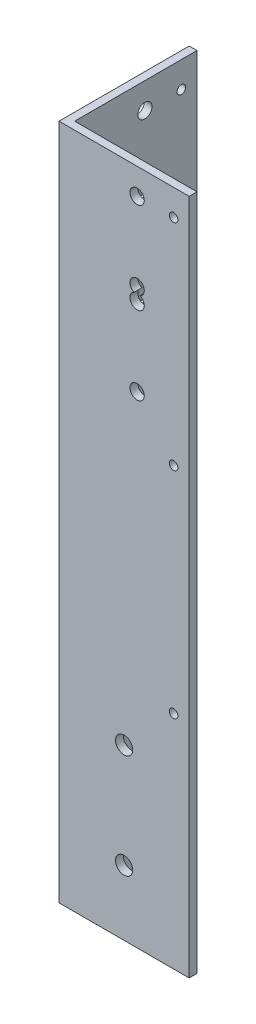
SolidWorks part; units mm, degrees
material "6061Al"
ref_plane "前视基准面" through (0, 0, 0) normal (0, 0, 1) x (1, 0, 0)
ref_plane "上视基准面" through (0, 0, 0) normal (0, 1, 0) x (1, 0, 0)
ref_plane "右视基准面" through (0, 0, 0) normal (1, 0, 0) x (0, 0, -1)
sketch "草图1" plane through (0, 0, 0) normal (0, 1, 0) x (1, 0, 0)
  line L0 (0, 0) -> (50, 0)
  line L1 (0, 0) -> (0, 50)
  line L2 (3, 3) -> (3, 50)
  line L3 (3, 3) -> (50, 3)
  line L4 (0, 50) -> (3, 50)
  line L5 (50, 3) -> (50, 0)
  dimension "D1" = 50
  dimension "D2" = 50
  dimension "D3" = 3
extrude "凸台-拉伸1" add sketch "草图1" along normal blind 260
hole_wizard "M5 间隙孔1" positions "草图2" profile "草图3" hole size "M5" standard "ISO" end condition through all
sketch "草图2" plane through (0, 0, -3) normal (0, 0, -1) x (-1, 0, 0)
  line L0 (-30, 215) -> (-30, 185) construction
  line L1 (-50, 260) -> (-50, 0) construction
  line L2 (-50, 260) -> (-3, 260) construction
  point P0 (-30, 250)
  point P3 (-30, 215)
  point P11 (-30, 220)
  point P12 (-30, 185)
  dimension "D2" = 30
  dimension "D3" = 35
  dimension "D5" = 20
  dimension "D6" = 10
  dimension "D1" = 2
sketch "草图3" plane through (30, 250, -3) normal (1, 0, 0) x (0, 1, 0)
  line L0 (0, 0) -> (0, 3)
  line L1 (0, 3) -> (2.75, 3)
  line L2 (2.75, 3) -> (2.75, 0)
  line L5 (2.75, 0) -> (0, 0)
  line L11 (0, -6.35) -> (0, 107.95) construction
  dimension "通孔孔直径" = 5.5
  dimension "通孔孔深度" = 3
hole_wizard "M5 间隙孔2" positions "草图4" profile "草图5" hole size "M5" standard "ISO" end condition through all
sketch "草图4" plane through (3, 0, 0) normal (1, 0, 0) x (0, 0, -1)
  line L0 (30, 185) -> (30, 215) construction
  line L1 (50, 260) -> (50, 0) construction
  line L2 (3, 260) -> (50, 260) construction
  point P0 (30, 220)
  point P3 (30, 185)
  point P12 (30, 250)
  point P13 (30, 215)
  dimension "D2" = 30
  dimension "D3" = 30
  dimension "D4" = 35
  dimension "D5" = 20
  dimension "D6" = 10
  dimension "D1" = 2
sketch "草图5" plane through (3, 220, -30) normal (0, 1, 0) x (0, 0, -1)
  line L0 (0, 0) -> (0, 3)
  line L1 (0, 3) -> (2.75, 3)
  line L2 (2.75, 3) -> (2.75, 0)
  line L5 (2.75, 0) -> (0, 0)
  line L11 (0, -6.35) -> (0, 107.95) construction
  dimension "通孔孔直径" = 5.5
  dimension "通孔孔深度" = 3
hole_wizard "M6 间隙孔1" positions "草图6" profile "草图7" hole size "M6" standard "ISO" end condition through all
sketch "草图6" plane through (0, 0, 0) normal (0, 0, 1) x (1, 0, 0)
  line L0 (25, 0) -> (25, 122.754) construction
  line L1 (0, 0) -> (50, 0) construction
  line L3 (25, 65) -> (25, 25) construction
  line L5 (25, 45) -> (97.4054, 45) construction
  point P2 (25, 65)
  point P6 (25, 25)
  dimension "D1" = 45
  dimension "D3" = 40
sketch "草图7" plane through (25, 65, 0) normal (1, 0, 0) x (0, -1, 0)
  line L0 (0, 0) -> (0, 50)
  line L1 (0, 50) -> (3.3, 50)
  line L2 (3.3, 50) -> (3.3, 0)
  line L5 (3.3, 0) -> (0, 0)
  line L11 (0, -6.35) -> (0, 107.95) construction
  dimension "通孔孔直径" = 6.6
  dimension "通孔孔深度" = 50
hole_wizard "M6 间隙孔2" positions "草图8" profile "草图9" hole size "M6" standard "ISO" end condition through all
sketch "草图8" plane through (0, 0, 0) normal (-1, 0, 0) x (0, 0, 1)
  line L0 (-25, 65) -> (-25, 25) construction
  line L2 (-25, 45) -> (-50, 45) construction
  line L3 (-50, 260) -> (-50, 0) construction
  line L5 (-50, 0) -> (0, 0) construction
  line L6 (-25, 0) -> (-25, 161.0792) construction
  point P0 (-25, 65)
  point P4 (-25, 25)
  dimension "D1" = 45
  dimension "D2" = 40
sketch "草图9" plane through (0, 65, -25) normal (0, 1, 0) x (0, 0, 1)
  line L0 (0, 0) -> (0, 50)
  line L1 (0, 50) -> (3.3, 50)
  line L2 (3.3, 50) -> (3.3, 0)
  line L5 (3.3, 0) -> (0, 0)
  line L11 (0, -6.35) -> (0, 107.95) construction
  dimension "通孔孔直径" = 6.6
  dimension "通孔孔深度" = 50
hole_wizard "M4 螺纹孔1" positions "草图10" profile "草图11" tap size "M4" standard "ISO" end condition through all
sketch "草图10" plane through (0, 0, -3) normal (0, 0, -1) x (-1, 0, 0)
  line L0 (-48.9, 250) -> (-39.1, 250)
  line L2 (-48.9, 167.5) -> (-39.1, 167.5)
  line L4 (-48.9, 85) -> (-39.1, 85)
  arc A0 (-46.5, 252.4) -> (-46.5, 247.6) centre (-46.5, 250) ccw construction
  arc A1 (-41.5, 247.6) -> (-41.5, 252.4) centre (-41.5, 250) ccw construction
  arc A2 (-46.5, 169.9) -> (-46.5, 165.1) centre (-46.5, 167.5) ccw construction
  arc A3 (-41.5, 165.1) -> (-41.5, 169.9) centre (-41.5, 167.5) ccw construction
  arc A4 (-46.5, 87.4) -> (-46.5, 82.6) centre (-46.5, 85) ccw construction
  arc A5 (-41.5, 82.6) -> (-41.5, 87.4) centre (-41.5, 85) ccw construction
  point P0 (-44, 250)
  point P2 (-44, 167.5)
  point P4 (-44, 85)
sketch "草图11" plane through (44, 250, -3) normal (1, 0, 0) x (0, 1, 0)
  line L0 (0, 0) -> (0, 3)
  line L1 (0, 3) -> (1.65, 3)
  line L2 (1.65, 3) -> (1.65, 0)
  line L5 (1.65, 0) -> (0, 0)
  line L11 (0, -6.35) -> (0, 107.95) construction
  dimension "通孔螺纹孔钻头直径" = 3.3
  dimension "通孔螺纹孔钻头深度" = 3
cosmetic thread "孔螺蚊线1" parameters "D2"=4
cosmetic thread "孔螺蚊线2" parameters "D2"=4
cosmetic thread "孔螺蚊线7" parameters "D2"=4
pattern_circular "阵列(圆周)1" [suppressed] count 2 over 90
hole_wizard "M4 螺纹孔2" positions "草图12" profile "草图13" tap size "M4" standard "ISO" end condition through all
sketch "草图12" plane through (3, 0, 0) normal (1, 0, 0) x (0, 0, -1)
  line L0 (44, 250) -> (44, 167.5) construction
  line L1 (50, 260) -> (50, 0) construction
  line L2 (3, 260) -> (50, 260) construction
  point P0 (44, 250)
  point P7 (44, 167.5)
  point P8 (44, 85)
  dimension "D2" = 82.5
  dimension "D3" = 6
  dimension "D4" = 10
  dimension "D1" = 3
sketch "草图13" plane through (3, 250, -44) normal (0, 1, 0) x (0, 0, -1)
  line L0 (0, 0) -> (0, 3)
  line L1 (0, 3) -> (1.65, 3)
  line L2 (1.65, 3) -> (1.65, 0)
  line L5 (1.65, 0) -> (0, 0)
  line L11 (0, -6.35) -> (0, 107.95) construction
  dimension "通孔螺纹孔钻头直径" = 3.3
  dimension "通孔螺纹孔钻头深度" = 3
cosmetic thread "孔螺蚊线5" parameters "D2"=4
cosmetic thread "孔螺蚊线6" parameters "D2"=4
cosmetic thread "孔螺蚊线8" parameters "D2"=4
